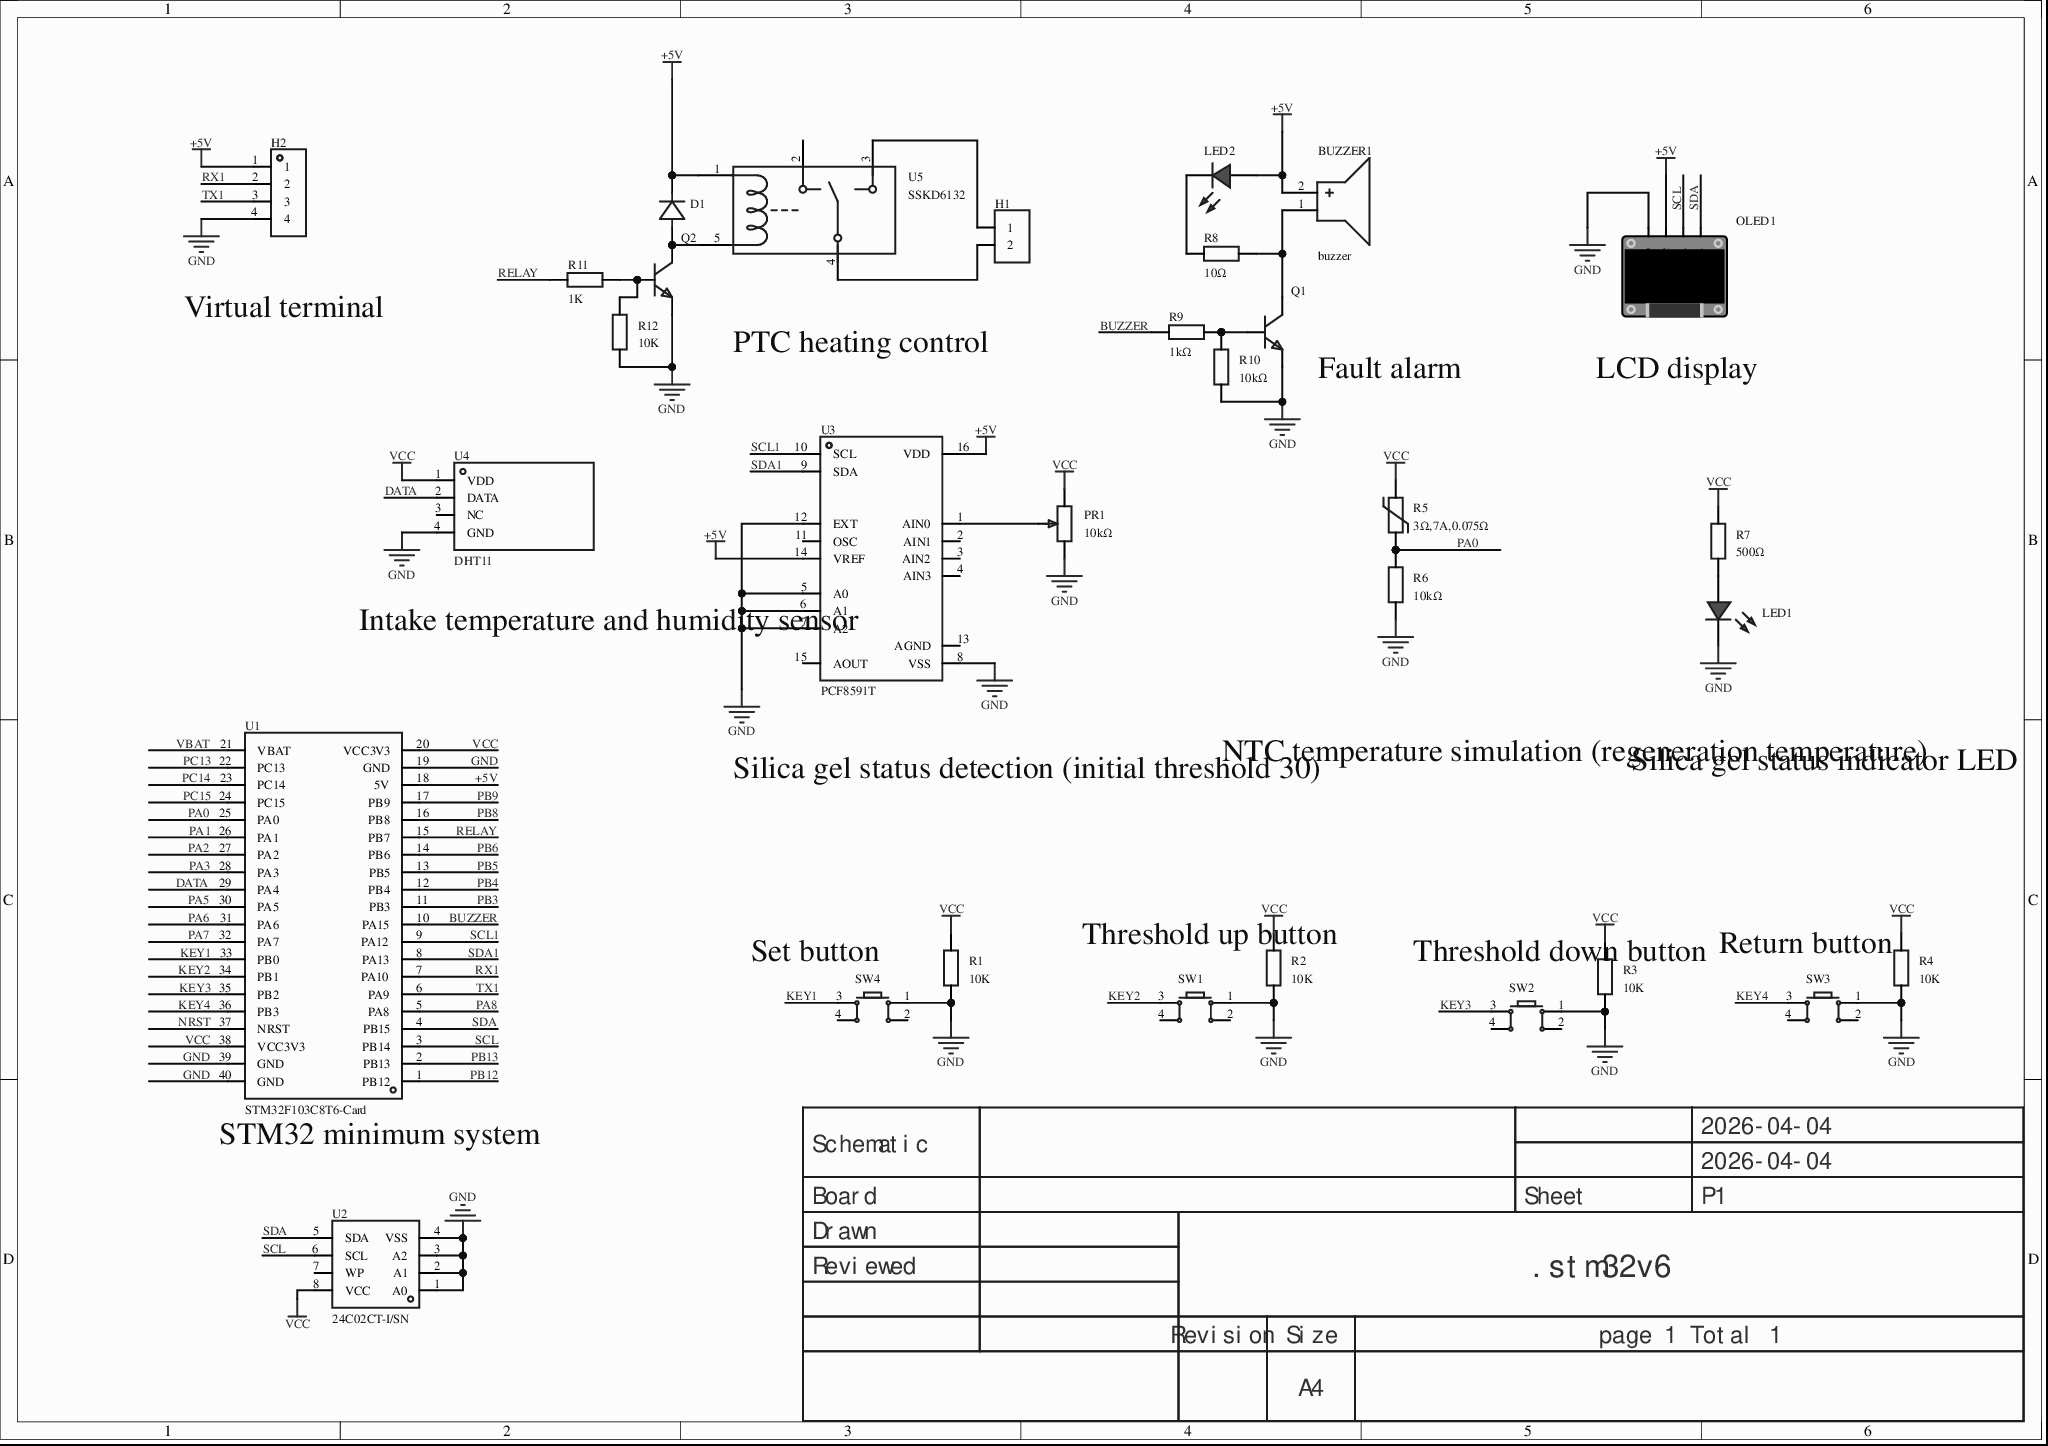
[diagram p0: MISC75094-3.schdoc]
# Altium project MISC75094-2.PrjPcb
1 sheet, 31 parts. Net scope: global (net labels, ports and power ports of the same name join across sheets).
Board file: MISC75094.pcbdoc

## Sheet MISC75094-3.schdoc
size 297 x 209 mm; Version: V1.0; @Project Name: MISC75094; @Page Count: 1; @Update Date: 2026-04-04; @Create Date: 2026-04-04; @Schematic Name: MISC75094; @Page No: 1; @Create Time: 23:22:16; @Update Time: 17:32:40; @Board Name: MISC75094

### Parts
BUZZER1  buzzer  [BUZ-TH_BD12.0-P6.00-D0.9-RD]
D1  (no value)  [DO_1N4007]
H1  (no value)  [HDR-TH_2P-P2.54-V-F]
H2  (no value)  [HDR-TH_4P-P2.54-V-F]
LED1  (no value)  [LED_TH-3mm]
LED2  (no value)  [LED_TH-3mm]
OLED1  (no value)  [0.96OLED_4P]
PR1  10kΩ  [R_3296]
Q1  (no value)  [S8050_TO_92]
Q2  (no value)  [S8050_TO_92]
R1  10K  [R0603]
R2  10K  [R0603]
R3  10K  [R0603]
R4  10K  [R0603]
R5  3Ω,7A,0.075Ω  [RES-TH_L16.5-W7.0-P7.50-D0.8-S6.2]
R6  10kΩ  [Res_1/8W]
R7  500Ω  [Res_1/8W]
R8  10Ω  [Res_1/8W]
R9  1kΩ  [Res_1/8W]
R10  10kΩ  [Res_1/8W]
R11  1K  [R0603]
R12  10K  [R0603]
SW1  (no value)  [SW-TH_4P-L6.0-W6.0-P4.50-LS6.5]
SW2  (no value)  [SW-TH_4P-L6.0-W6.0-P4.50-LS6.5]
SW3  (no value)  [SW-TH_4P-L6.0-W6.0-P4.50-LS6.5]
SW4  (no value)  [SW-TH_4P-L6.0-W6.0-P4.50-LS6.5]
U1  STM32F103C8T6-Card  [CONN-TH_L53.3-W22.9_STM32F103C8T6-CARD]
U2  24C02CT-I/SN  [SOIC-8_L4.9-W3.9-P1.27-LS6.0-BL]
U3  PCF8591T  [SOIC-16_L10.3-W7.5-P1.27-LS10.3-BL]
U4  DHT11  [SENSOR-TH_DHT11]
U5  SSKD6132  [RELAY-TH_G2R-1]

### Nets
+5V: BUZZER1.2(+) D1.1(K) H2.1 LED2.1(C) OLED1.2(VCC) U1.18(5V) U3.14(VREF) U3.16(VDD) U5.1
GND: H2.4 LED1.2(A) OLED1.1(GND) PR1.3 Q1.1(E) Q2.1(E) R1.1 R2.1 R3.1 R4.1 R6.1 R10.1 R12.1 SW1.1 SW2.1 SW3.1 SW4.1 U1.19(GND) U1.39(GND) U1.40(GND) U2.1(A0) U2.2(A1) U2.3(A2) U2.4(VSS) U3.5(A0) U3.6(A1) U3.7(A2) U3.8(VSS) U3.12(EXT) U4.4(GND)
VCC: PR1.1 R1.2 R2.2 R3.2 R4.2 R5.2 R7.2 U1.20(VCC3V3) U1.38(VCC3V3) U2.8(VCC) U4.1(VDD)
BUZZER: R9.1 U1.10(PA15)
DATA: U1.29(PA4) U4.2(DATA)
KEY1: SW4.3 U1.33(PB0)
KEY2: SW1.3 U1.34(PB1)
KEY3: SW2.3 U1.35(PB2)
KEY4: SW3.3 U1.36(PB3)
NRST: U1.37(NRST)
PA0: R5.1 R6.2 U1.25(PA0)
PA1: U1.26(PA1)
PA2: U1.27(PA2)
PA3: U1.28(PA3)
PA5: U1.30(PA5)
PA6: U1.31(PA6)
PA7: U1.32(PA7)
PA8: U1.5(PA8)
PB3: U1.11(PB3)
PB4: U1.12(PB4)
PB5: U1.13(PB5)
PB6: U1.14(PB6)
PB8: U1.16(PB8)
PB9: U1.17(PB9)
PB12: U1.1(PB12)
PB13: U1.2(PB13)
PC13: U1.22(PC13)
PC14: U1.23(PC14)
PC15: U1.24(PC15)
RELAY: R11.1 U1.15(PB7)
RX1: H2.2 U1.7(PA10)
SCL: OLED1.3(SCL) U1.3(PB14) U2.6(SCL)
SCL1: U1.9(PA12) U3.10(SCL)
SDA: OLED1.4(SDA) U1.4(PB15) U2.5(SDA)
SDA1: U1.8(PA13) U3.9(SDA)
TX1: H2.3 U1.6(PA9)
VBAT: U1.21(VBAT)
NetBUZZER1_1: BUZZER1.1(-) Q1.3(C) R8.1
NetD1_2: D1.2(A) Q2.3(C) U5.5
NetH1_1: H1.1 U5.3
NetH1_2: H1.2 U5.4
NetLED1_1: LED1.1(C) R7.1
NetLED2_2: LED2.2(A) R8.2
NetPR1_2: PR1.2 U3.1(AIN0)
NetQ1_2: Q1.2(B) R9.2 R10.2
NetQ2_2: Q2.2(B) R11.2 R12.2

Not connected (* = marked no-connect by the designer): SW1 2 4; SW2 2 4; SW3 2 4; SW4 2 4; U2 7(WP); U3 2(AIN1) 3(AIN2) 4(AIN3) 11(OSC) 13(AGND) 15(AOUT); U4 3(NC); U5 2

### Notes on the sheet
- Virtual terminal
- PTC heating control
- (near Q1) Fault alarm
- LCD display
- (near U3) Intake temperature and humidity sensor
- Silica gel status detection (initial threshold 30)
- NTC temperature simulation (regeneration temperature)
- Silica gel status indicator LED
- (near R2) Threshold up button
- (near R4) Return button
- Set button
- (near R3) Threshold down button
- (near U1) STM32 minimum system
- 2026-04-04
- Schematic
- Board
- Sheet
- P1
- Drawn
- Reviewed
- .stm32v6
- Revision
- Size
- A4
- page 1 Total 1

### Library data of the parts
BUZZER1 = buzzer: AddInBom: yes; ModelId: af17e4151ed84fc2a628230bf23763630819f05c4eef4c71ace90d822a990e87; ModelTransform: 472.44,472.176,0,270,0,0,0,0,-196.85; Symbol: BUZZER; Device: buzzer; LCSC Part Name: buzzer; SupplierPart: C9900014030; ManufacturerPart: buzzer; Supplier Footprint: buzzer; JLCPCB Part Class: Extended Part; Supplier: LCSC; ConvertToPcb: yes; FootprintName: BUZ-TH_BD12.0-P6.00-D0.9-RD; ModelName: BUZ-TH_BD12.0-P6.00-D0.9-RD
D1 = D_1N4007A: AddInBom: yes; ModelId: 6de1e9b71a0d4751b4e9df530304c1a30819f05c4eef4c71ace90d822a990e87; ModelName: DO-41_D2.4-L4.7-P8.70; ModelTransform: 373.9,94.4,232.29,0,0,0,0,0,-140; Symbol: D_1N4007; Device: D_1N4007A; Supplier Footprint: DO-41; ConvertToPcb: yes; FootprintName: DO_1N4007
H1 = HDR-F_2.54_1x2P: Symbol: Header-Female-2.54_1x2; ConvertToPcb: yes; ModelId: a9450ef445564560a104363b9aacde4e; ModelName: HDR-TH_2P-P2.54-F-LI-1X2P; ModelTransform: 215.7476,98.425,0,0,0,0,0,0,-129.921; Device: HDR-F_2.54_1x2P; AddInBom: yes; SupplierPart: C49661; Supplier Footprint: 插件; FootprintName: HDR-TH_2P-P2.54-V-F
H2 = HDR-F_2.54_1x4P: Symbol: 2.54-1*4P female; 3D Model: d187812051054f85879fcaa51a310d8e0819f05c4eef4c71ace90d822a990e87; 3D Model Transform: 419.6842,98.464,0,0,0,0,0,0,-118.11; ConvertToPcb: yes; Device: HDR-F_2.54_1x4P; Supplier Part: C2718488; Supplier Footprint: 插件; AddInBom: yes; FootprintName: HDR-TH_4P-P2.54-V-F; ModelName: HDR-TH_4P-P2.54-V-F
LED1 LED2 = LED_TH-R_3mm: ConvertToPcb: yes; ModelId: a497c992633541038a38947cdc58012f0819f05c4eef4c71ace90d822a990e87; ModelName: LED-TH-3mm_R; ModelTransform: 141.274,153.327,0,0,0,0,-5.984,0,-137.795; Symbol: LED_TH-R; Device: LED_TH-R_3mm; AddInBom: yes; FootprintName: LED_TH-3mm; Supplier Footprint: 插件
OLED1 = 0.96OLED模块_4P: Symbol: 0.96OLED module_4P; ConvertToPcb: yes; ModelId: 79c000fdb68d45a296c2e9bedf4f9055; ModelTransform: 1393.69792,1318.895,0,0,0,0,0,-560.079,-137.795; Device: 0.96OLED module_4P; AddInBom: yes; FootprintName: 0.96OLED_4P; Supplier Footprint: 插件; ModelName: 0.96OLED_4P
PR1 = R_3296: ConvertToPcb: yes; ModelId: b182808559bb43bda9e7de64b64134cb; ModelName: 3296W; ModelTransform: 373.98,188.96,590.49,180,0,0,0,0,-140; Symbol: R_3296; Device: R_3296; AddInBom: yes; Supplier Footprint: 直插; FootprintName: R_3296; Value: 10kΩ
Q1 Q2 = S8050_TO_NPN: ConvertToPcb: yes; ModelId: aafe8e06f2154e7c93506efd0d6632dd; ModelName: TO-92-3_L4.9-W3.7-P1.27-L; ModelTransform: 180.78,141.44,417.3,0,0,0,0,0,-200; Symbol: S8050_TO_NPN; Device: S8050_TO_NPN; AddInBom: yes; Supplier Footprint: TO-92; FootprintName: S8050_TO_92
R1-R4 R11 R12 = Res_0603: Symbol: Resistor; ConvertToPcb: yes; ModelId: fc143cca1e79419f9cd78b61e9279f080819f05c4eef4c71ace90d822a990e87; ModelTransform: 31.8897,63.7794,0,90,0,0,0,0,0; Device: Res_0603; AddInBom: yes; Supplier Footprint: 0603; FootprintName: R0603; ModelName: R0603
  R1-R4 R12: Value: 10K
  R11: Value: 1K
R5 = 3Ω,7A,0.075Ω: AddInBom: yes; ModelId: 8a9841f8c9dc4c8dbe0b05dff75b51ae0819f05c4eef4c71ace90d822a990e87; ModelTransform: 649.426,314.96,0,0,0,0,0,0,-196.85; Symbol: 3Ω,7A,0.075Ω; Device: 3Ω,7A,0.075Ω; LCSC Part Name: 3Ω,7A,0.075Ω; SupplierPart: C9900017035; ManufacturerPart: 3Ω,7A,0.075Ω; Supplier Footprint: NTC_15D; JLCPCB Part Class: Extended Part; Supplier: LCSC; ConvertToPcb: yes; FootprintName: RES-TH_L16.5-W7.0-P7.50-D0.8-S6.2; ModelName: RES-TH_L16.5-W7.0-P7.50-D0.8-S6.2
R6-R10 = Res_AXIAL-1/8W: Symbol: Resistor; ConvertToPcb: yes; ModelId: b2b5ae7ae4c642178fe0039925c86a3f0819f05c4eef4c71ace90d822a990e87; ModelName: RES-TH_BD1.8-L3.2-P7.20-D0.4; ModelTransform: 282.86,66.88,253.09,0,0,0,0,0,-191; Device: Res_AXIAL-1/8W; AddInBom: yes; Supplier Footprint: 轴向引线; FootprintName: Res_1/8W
  R6 R10: Value: 10kΩ
  R7: Value: 500Ω
  R8: Value: 10Ω
  R9: Value: 1kΩ
SW1-SW3 = Key_TH_6x6x6: Contact current: 50mA; rated voltage (DC): 12V; insulation resistance: 100MΩ; circuit: SPST; mounting: through-hole; button shape: round; button/cap colour: black; force: 260gf@±30gf; operating temperature: -25℃~+70℃; pin style: PC pin; switch length: 6mm; switch width: 6mm; switch height: 6mm; with bracket: no;; Symbol: Tactile switch; 3D Model: 20eee248bc684ccd8cbdbb1d0d91ec6f0819f05c4eef4c71ace90d822a990e87; 3D Model Transform: 236.22,323.03,0,90,0,0,0,0,-137.795; AddInBom: yes; ModelName: SW-TH_4P-L6.0-W6.0-H5.0-LS6.5-P4.50; Device: Key_TH_6x6x6; Supplier Footprint: 插件; ConvertToPcb: yes; FootprintName: SW-TH_4P-L6.0-W6.0-P4.50-LS6.5
SW4 = Key_TH_6x6x6: Contact current: 50mA; rated voltage (DC): 12V; insulation resistance: 100MΩ; circuit: SPST; mounting: through-hole; button shape: round; button/cap colour: black; force: 260gf@±30gf; operating temperature: -25℃~+70℃; pin style: PC pin; switch length: 6mm; switch width: 6mm; switch height: 6mm; with bracket: no;; Symbol: Tactile switch; AddInBom: yes; ModelId: 20eee248bc684ccd8cbdbb1d0d91ec6f0819f05c4eef4c71ace90d822a990e87; ModelName: SW-TH_4P-L6.0-W6.0-H5.0-LS6.5-P4.50; ModelTransform: 236.22,323.03,0,90,0,0,0,0,-137.795; Device: Key_TH_6x6x6; ConvertToPcb: yes; FootprintName: SW-TH_4P-L6.0-W6.0-P4.50-LS6.5; Supplier Footprint: 插件
U1 = STM32F103C8T6-Card: AddInBom: yes; Symbol: STM32F103C8T6-CARD; Device: STM32F103C8T6-Card; LCSC Part Name: STM32F103C8T6-Card; SupplierPart: C9900077949; ManufacturerPart: STM32F103C8T6-Card; Supplier Footprint: 插件; Supplier: LCSC; ConvertToPcb: yes; FootprintName: CONN-TH_L53.3-W22.9_STM32F103C8T6-CARD
U2 = 24C02CT-I/SN: Interface type: I2C; storage capacity: 2Kbit; clock frequency (fc): 400kHz;; AddInBom: yes; ModelId: e81d2f7d937b4a6ab1dca543ff5d56a40819f05c4eef4c71ace90d822a990e87; ModelName: SOIC-8_L4.9-W3.9-H1.7-LS6.0-P1.27; ModelTransform: 192.913,236.22,0,0,0,0,0,0,0; Supply Voltage: 4.5V~5.5V; Write Cycle Time (Tw): 1ms; Symbol: 24C02CT-I/SN; Device: 24C02CT-I/SN; LCSC Part Name: 24C02CT-I/SN; SupplierPart: C2061172; ManufacturerPart: 24C02CT-I/SN; Supplier Footprint: SOIC-8; JLCPCB Part Class: Extended Part; Supplier: LCSC; ConvertToPcb: yes; FootprintName: SOIC-8_L4.9-W3.9-P1.27-LS6.0-BL; Interface Type: I2C; Memory Size: 2Kbit; Clock Frequency (fc): 400kHz; Operating Temperature: -40℃~+85℃
U3 = PCF8591T: Manufacturer: NXP(恩智浦); Symbol: PCF8591T_C26984142; AddInBom: yes; ModelId: 2da8125c657e49328ba6fa7b098653dd0819f05c4eef4c71ace90d822a990e87; ModelName: SOIC-16_L10.3-W7.5-H2.7-LS10.3-P1.27; ModelTransform: 405.511,409.68154,0,0,0,0,-0.0005,0,0; Device: PCF8591T; LCSC Part Name: PCF8591T; SupplierPart: C26984142; ManufacturerPart: PCF8591T; Supplier Footprint: -; JLCPCB Part Class: Extended Part; Supplier: LCSC; ConvertToPcb: yes; FootprintName: SOIC-16_L10.3-W7.5-P1.27-LS10.3-BL
U4 = DHT11: New capacitive digital temperature and humidity sensor; old model discontinued; 16.1x12.6x5.8mm; Manufacturer: 广州奥松; AddInBom: yes; ModelId: 6dde47d4d8bf4fa598dffcc067449c1d; ModelTransform: 236.25937,492.125,0,270,0,0,0,-11.811,-196.85; Symbol: DHT11; Device: DHT11; LCSC Part Name: 新款电容式数字温湿度传感器,老款已停产16.1x12.6x5.8mm DHT11  电容式传感器; SupplierPart: C117051; ManufacturerPart: DHT11; Supplier Footprint: SIP-4; JLCPCB Part Class: Extended library; Datasheet: https://example.com/20170703/1499081238365.pdf; Supplier: LCSC; ConvertToPcb: yes; FootprintName: SENSOR-TH_DHT11; ModelName: SENSOR-TH_DHT11
U5 = SSKD6132: AddInBom: yes; ModelId: fe99462dd15043c98af5adb0e5338dda0819f05c4eef4c71ace90d822a990e87; ModelTransform: 1141.73,511.81,0,0,0,0,26.417,-0.354,-157.48; Symbol: SSKD6132; Device: SSKD6132; LCSC Part Name: SSKD6132; SupplierPart: C9900012103; ManufacturerPart: SSKD6132; Supplier Footprint: RELAY-TH_G2R-1; JLCPCB Part Class: Extended Part; Supplier: LCSC; ConvertToPcb: yes; FootprintName: RELAY-TH_G2R-1; ModelName: RELAY-TH_G2R-1